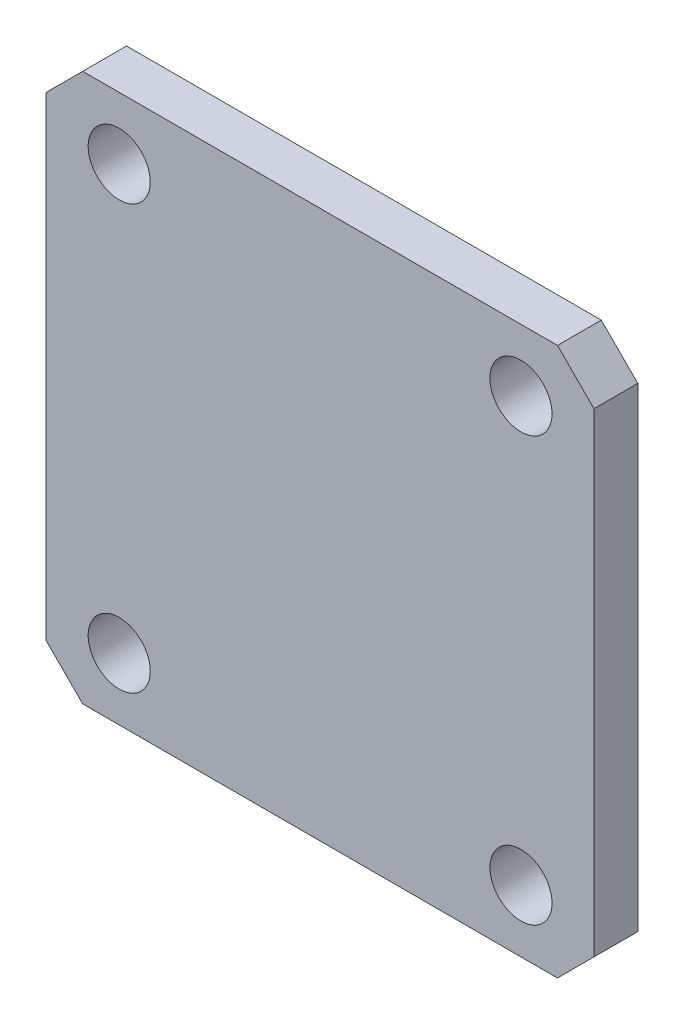
SolidWorks part; units mm, degrees
material "1023 碳钢板 (SS)"
ref_plane "Front Plane" through (0, 0, 0) normal (0, 0, 1) x (1, 0, 0)
ref_plane "Top Plane" through (0, 0, 0) normal (0, 1, 0) x (1, 0, 0)
ref_plane "Right Plane" through (0, 0, 0) normal (1, 0, 0) x (0, 0, -1)
sketch "Sketch1" plane through (0, 0, 0) normal (0, 0, 1) x (1, 0, 0)
  line L0 (-37.5, 32.5) -> (-32.5, 37.5)
  line L1 (-32.5, 37.5) -> (32.5, 37.5)
  line L2 (-37.5, 32.5) -> (-37.5, -32.5)
  line L3 (-32.5, -37.5) -> (32.5, -37.5)
  line L4 (37.5, 32.5) -> (37.5, -32.5)
  line L5 (-37.5, 37.5) -> (37.5, -37.5) construction
  line L6 (-37.5, -37.5) -> (37.5, 37.5) construction
  line L7 (32.5, 37.5) -> (37.5, 32.5)
  line L8 (32.5, -37.5) -> (37.5, -32.5)
  line L9 (-37.5, -32.5) -> (-32.5, -37.5)
  line L10 (-27.5, 29) -> (-27.5, -29) construction
  line L11 (-27.5, 29) -> (27.5, 29) construction
  line L13 (-27.5, -29) -> (27.5, -29) construction
  line L14 (27.5, 29) -> (27.5, -29) construction
  line L15 (-27.5, 29) -> (27.5, -29) construction
  line L16 (-27.5, -29) -> (27.5, 29) construction
  circle A0 centre (-27.5, 29) radius 4.25
  circle A1 centre (27.5, 29) radius 4.25
  circle A2 centre (-27.5, -29) radius 4.25
  circle A3 centre (27.5, -29) radius 4.25
  point P0 (0, 0)
  point P14 (0, 0)
  dimension "D4" = 8.5
  dimension "D1" = 75
  dimension "D2" = 75
  dimension "D3" = 58
  dimension "D9" = 55
extrude "Boss-Extrude1" add sketch "Sketch1" along normal blind 6
